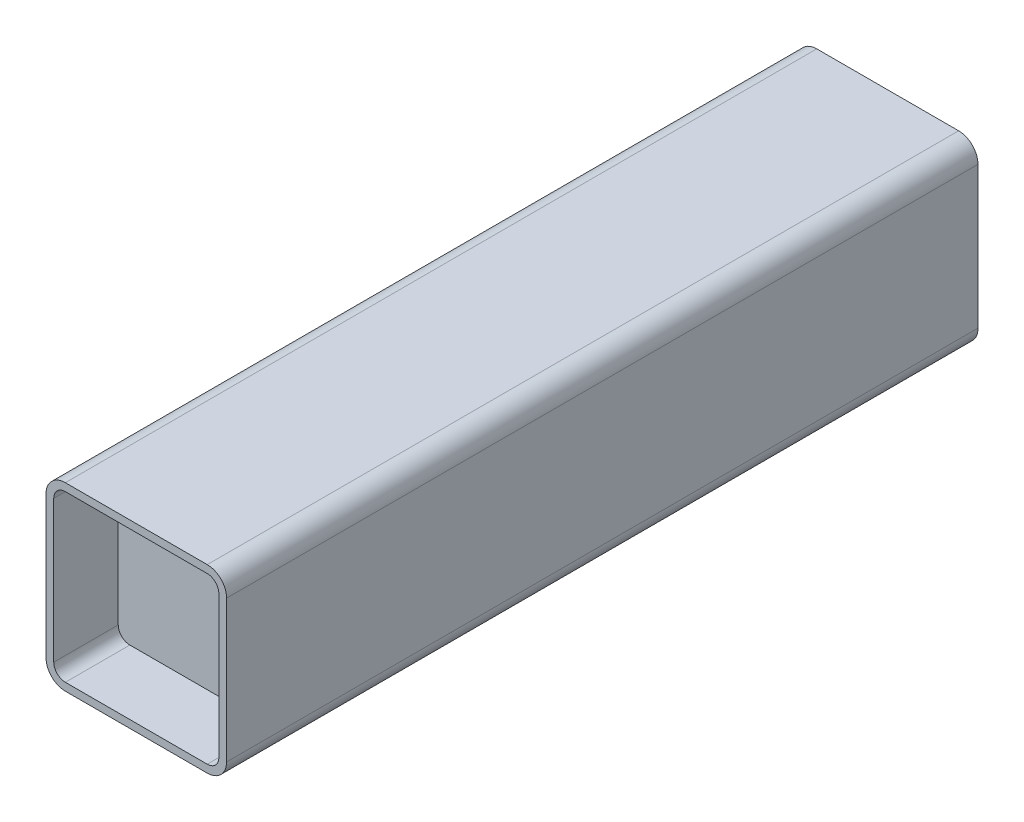
SolidWorks part; units mm, degrees
material "Q345"
ref_plane "前视基准面" through (0, 0, 0) normal (0, 0, 1) x (1, 0, 0)
ref_plane "上视基准面" through (0, 0, 0) normal (0, 1, 0) x (1, 0, 0)
ref_plane "右视基准面" through (0, 0, 0) normal (1, 0, 0) x (0, 0, -1)
sketch "草图1" plane through (0, 0, 0) normal (0, 0, 1) x (1, 0, 0)
  line L0 (-110, 128) -> (110, 128)
  line L1 (-110, 140) -> (110, 140)
  line L2 (-140, 110) -> (-140, -110)
  line L3 (-110, -140) -> (110, -140)
  line L4 (140, 110) -> (140, -110)
  line L5 (-140, 140) -> (140, -140) construction
  line L6 (-140, -140) -> (140, 140) construction
  line L7 (128, 110) -> (128, -110)
  line L8 (-110, -128) -> (110, -128)
  line L9 (-128, 110) -> (-128, -110)
  arc A0 (110, -140) -> (140, -110) centre (110, -110) ccw
  arc A1 (-110, -140) -> (-140, -110) centre (-110, -110) cw
  arc A2 (140, 110) -> (110, 140) centre (110, 110) ccw
  arc A3 (-140, 110) -> (-110, 140) centre (-110, 110) cw
  arc A4 (128, 110) -> (110, 128) centre (110, 110) ccw
  arc A5 (110, -128) -> (128, -110) centre (110, -110) ccw
  arc A6 (-110, -128) -> (-128, -110) centre (-110, -110) cw
  arc A7 (-128, 110) -> (-110, 128) centre (-110, 110) cw
  point P0 (0, 0)
  dimension "D3" = 30
  dimension "D1" = 280
  dimension "D2" = 280
  dimension "D4" = 12
extrude "凸台-拉伸1" add sketch "草图1" along normal blind 1165
sketch "草图2" plane through (0, 0, 1165) normal (0, 0, 1) x (1, 0, 0)
  line L0 (128, -110) -> (128, 110) construction
  line L1 (-110, -128) -> (110, -128) construction
  line L2 (-128, 110) -> (-128, -110) construction
  line L3 (110, 128) -> (-110, 128) construction
  line L4 (128, -110) -> (128, 110)
  line L5 (-110, -128) -> (110, -128)
  line L6 (-128, 110) -> (-128, -110)
  line L7 (110, 128) -> (-110, 128)
  arc A0 (128, 110) -> (110, 128) centre (110, 110) ccw construction
  arc A1 (110, -128) -> (128, -110) centre (110, -110) ccw construction
  arc A2 (-128, -110) -> (-110, -128) centre (-110, -110) ccw construction
  arc A3 (-110, 128) -> (-128, 110) centre (-110, 110) ccw construction
  arc A4 (128, 110) -> (110, 128) centre (110, 110) ccw
  arc A5 (110, -128) -> (128, -110) centre (110, -110) ccw
  arc A6 (-128, -110) -> (-110, -128) centre (-110, -110) ccw
  arc A7 (-110, 128) -> (-128, 110) centre (-110, 110) ccw
extrude "凸台-拉伸2" add sketch "草图2" against normal blind 10 from offset 100 offset against normal yes
ref_plane "基准面1" through (0, 0, 582.5) normal (0, 0, 1) x (1, 0, 0)
mirror "镜向1" about plane through (0, 0, 582.5) normal (0, 0, 1) of "凸台-拉伸2"
sketch "草图4" plane through (0, -128, 0) normal (0, 1, 0) x (1, 0, 0)
  line L0 (-110, -1055) -> (110, -1055) construction
  line L3 (0, -110) -> (0, -1055) construction
  line L4 (128, -1055) -> (128, -110) construction
  line L5 (-128, -735) -> (128, -735)
  line L6 (-128, -735) -> (-128, -745)
  line L7 (-128, -745) -> (128, -745)
  line L8 (128, -735) -> (128, -745)
  line L9 (-128, -735) -> (128, -745) construction
  line L10 (-128, -745) -> (128, -735) construction
  line L11 (-110, -110) -> (110, -110) construction
  line L13 (-128, -430) -> (128, -430)
  line L14 (-128, -430) -> (-128, -420)
  line L15 (-128, -420) -> (128, -420)
  line L16 (128, -430) -> (128, -420)
  line L17 (-128, -430) -> (128, -420) construction
  line L18 (-128, -420) -> (128, -430) construction
  point P6 (0, -740)
  point P14 (0, -425)
  dimension "D1" = 10
  dimension "D2" = 315
  dimension "D3" = 10
  dimension "D4" = 315
extrude "凸台-拉伸4" add sketch "草图4" along normal up to surface (256 mm away) up to face at (0, 128, 50)
sketch "草图5" plane through (0, -128, 0) normal (0, 1, 0) x (1, 0, 0)
  line L0 (0, -1165) -> (0, 0) construction
  line L1 (-110, -1165) -> (110, -1165) construction
  line L2 (0, -582.5) -> (286.8876, -582.5) construction
  line L3 (0, -1125) -> (-80, -1125) construction
  circle A0 centre (0, -1125) radius 16
  circle A1 centre (0, -40) radius 16
  circle A2 centre (-80, -1125) radius 16
  circle A3 centre (80, -1125) radius 16
  circle A4 centre (80, -40) radius 16
  circle A5 centre (-80, -40) radius 16
  dimension "D1" = 32
  dimension "D2" = 1085
  dimension "D3" = 80
sketch "草图7" plane through (140, 0, 0) normal (1, 0, 0) x (0, 0, -1)
  line L0 (-240, 110) -> (-240, -110) construction
  line L3 (0, -110) -> (0, 110) construction
  line L4 (-430, 75) -> (-50, 75)
  line L5 (-430, 75) -> (-430, -75)
  line L6 (-430, -75) -> (-50, -75)
  line L7 (-50, 75) -> (-50, -75)
  line L8 (-430, 75) -> (-50, -75) construction
  line L9 (-430, -75) -> (-50, 75) construction
  line L10 (-1165, 110) -> (0, 110) construction
  line L11 (-1165, -110) -> (0, -110) construction
  point P6 (-240, 0)
  dimension "D1" = 380
  dimension "D2" = 150
  dimension "D3" = 50
